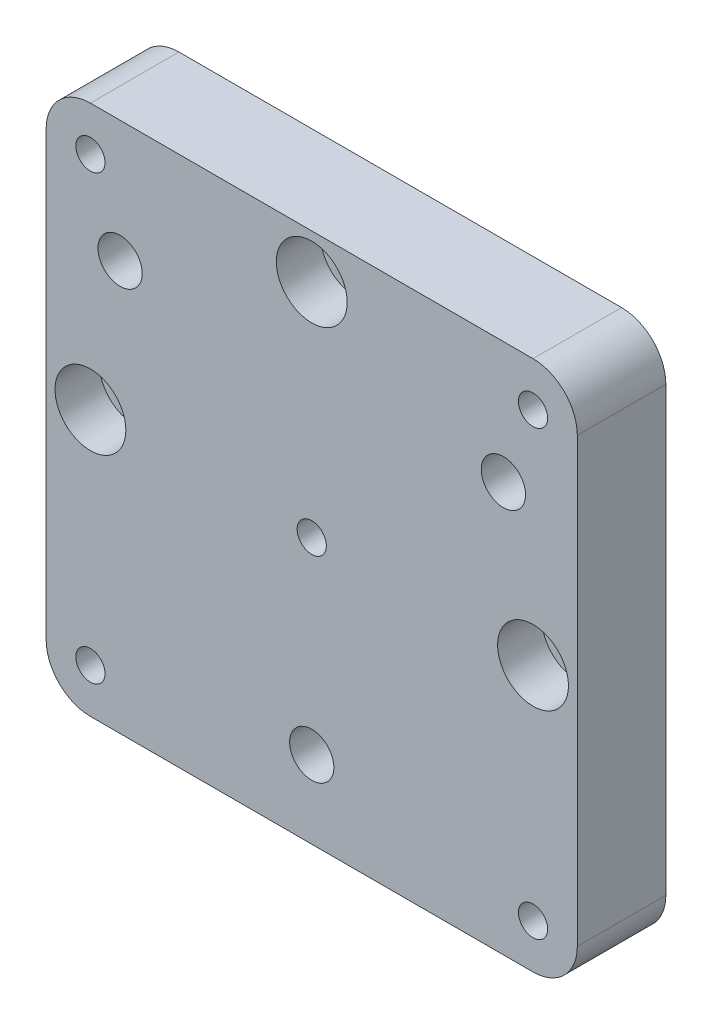
SolidWorks part; units mm, degrees
ref_plane "Front Plane" through (0, 0, 0) normal (0, 0, 1) x (1, 0, 0)
ref_plane "Top Plane" through (0, 0, 0) normal (0, 1, 0) x (1, 0, 0)
ref_plane "Right Plane" through (0, 0, 0) normal (1, 0, 0) x (0, 0, -1)
sketch "Sketch1" plane through (0, 0, 0) normal (0, 0, 1) x (1, 0, 0)
  line L1 (39.1638, -30) -> (-20.8362, -30)
  line L2 (39.1638, -30) -> (39.1638, 30)
  line L3 (39.1638, 30) -> (-20.8362, 30)
  line L4 (-20.8362, -30) -> (-20.8362, 30)
  line L5 (39.1638, -30) -> (-20.8362, 30) construction
  line L6 (39.1638, 30) -> (-20.8362, -30) construction
  point P0 (9.1638, 0)
  dimension "D1" = 60
extrude "Boss-Extrude1" add sketch "Sketch1" along normal blind 10
fillet "Fillet1" radius 5 4 edges at (-20.8362, 30, 5) (39.1638, 30, 5) (39.1638, -30, 5) (-20.8362, -30, 5)
hole_wizard "M6 Tapped Hole1" positions "Sketch6" profile "Sketch7" tap size "M6" standard "GB"
sketch "Sketch6" plane through (0, 0, 10) normal (0, 0, 1) x (1, 0, 0)
  point P0 (9.1638, -21.25)
  point P3 (30.8144, 16.25)
  point P6 (-12.4868, 16.25)
sketch "Sketch7" plane through (9.1638, -21.25, 10) normal (1, 0, 0) x (0, -1, 0)
  line L0 (0, 0) -> (0, 16.5022)
  line L1 (0, 16.5022) -> (2.5, 15)
  line L2 (2.5, 15) -> (2.5, 0)
  line L5 (2.5, 0) -> (0, 0)
  line L10 (0, 16.5022) -> (-2.5, 15) construction
  line L11 (0, -6.35) -> (0, 107.95) construction
  dimension "螺纹孔钻头直径" = 5
  dimension "螺纹孔钻头深度" = 15
  dimension "导头角度" = 118
cosmetic thread "Cosmetic Thread1"
cosmetic thread "Cosmetic Thread2"
cosmetic thread "Cosmetic Thread3"
sketch "Sketch8" plane through (0, 0, 10) normal (0, 0, 1) x (1, 0, 0)
  circle A0 centre (9.1638, 25) radius 2.1
  circle A1 centre (34.1638, 0) radius 2.1
  circle A2 centre (-15.8362, 0) radius 2.1
  dimension "D1" = 4.2
extrude "Cut-Extrude1" cut sketch "Sketch8" against normal through all
sketch "Sketch9" plane through (0, 0, 10) normal (0, 0, 1) x (1, 0, 0)
  circle A0 centre (-15.8362, 0) radius 4
  circle A1 centre (9.1638, 25) radius 4
  circle A2 centre (34.1638, 0) radius 4
  dimension "D1" = 8
extrude "Cut-Extrude2" cut sketch "Sketch9" against normal blind 5
hole_wizard "M4 Tapped Hole1" positions "Sketch10" profile "Sketch12" tap size "M4" standard "GB" end condition through all
sketch "Sketch10" plane through (0, 0, 10) normal (0, 0, 1) x (1, 0, 0)
  point P0 (-15.8362, -25)
  point P3 (34.1638, -25)
  point P6 (34.1638, 25)
  point P9 (-15.8362, 25)
sketch "Sketch12" plane through (-15.8362, -25, 10) normal (1, 0, 0) x (0, -1, 0)
  line L0 (0, 0) -> (0, 10)
  line L1 (0, 10) -> (1.65, 10)
  line L2 (1.65, 10) -> (1.65, 0)
  line L5 (1.65, 0) -> (0, 0)
  line L11 (0, -6.35) -> (0, 107.95) construction
  dimension "通孔螺纹孔钻头直径" = 3.3
  dimension "通孔螺纹孔钻头深度" = 10
cosmetic thread "Cosmetic Thread4"
cosmetic thread "Cosmetic Thread5"
cosmetic thread "Cosmetic Thread6"
cosmetic thread "Cosmetic Thread7"
hole_wizard "M4 Tapped Hole2" positions "Sketch13" profile "Sketch14" tap size "M4" standard "GB" end condition through all
sketch "Sketch13" plane through (0, 0, 10) normal (0, 0, 1) x (1, 0, 0)
  line L0 (-20.8362, 0) -> (39.1638, 0) construction
  line L1 (-20.8362, 25) -> (-20.8362, -25) construction
  line L2 (39.1638, -25) -> (39.1638, 25) construction
  point P11 (9.1638, 0)
sketch "Sketch14" plane through (9.1638, 0, 10) normal (1, 0, 0) x (0, -1, 0)
  line L0 (0, 0) -> (0, 10)
  line L1 (0, 10) -> (1.65, 10)
  line L2 (1.65, 10) -> (1.65, 0)
  line L5 (1.65, 0) -> (0, 0)
  line L11 (0, -6.35) -> (0, 107.95) construction
  dimension "通孔螺纹孔钻头直径" = 3.3
  dimension "通孔螺纹孔钻头深度" = 10
cosmetic thread "Cosmetic Thread8" parameters "D2"=4
